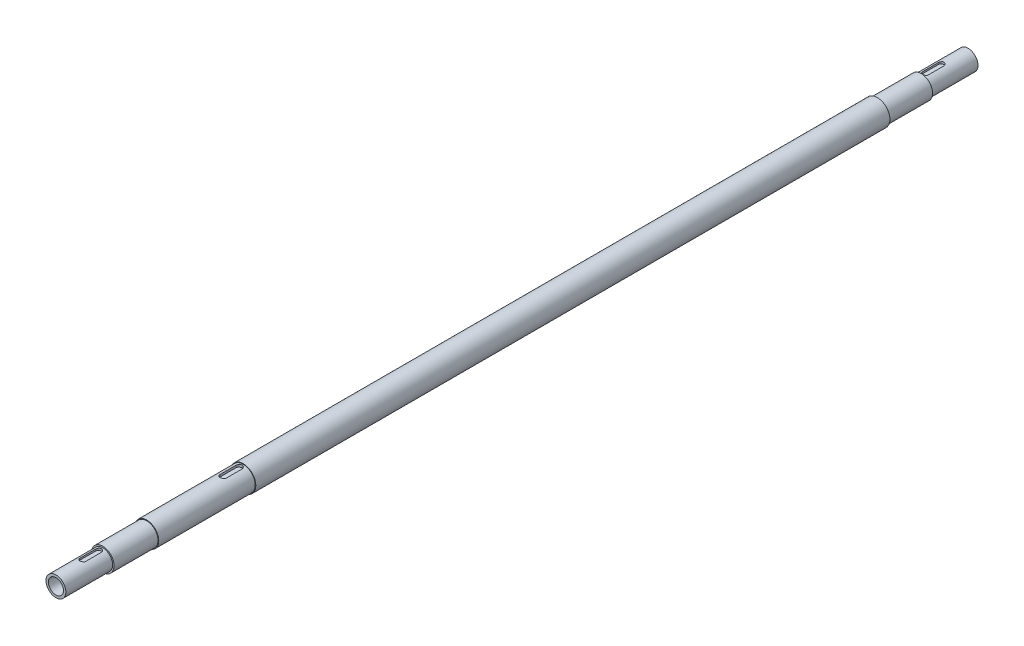
from build123d import *

# Parameters (mm, degrees)
SKETCH1_R           = 44.5
BOSS_EXTRUDE1_DEPTH = 3215
CUT_EXTRUDE1_START  = -165
SKETCH2_R           = 44.5
SKETCH2_R_2         = 37.5
CUT_EXTRUDE1_DEPTH  = 165
CUT_EXTRUDE2_START  = -155
SKETCH3_R           = 44.5
SKETCH3_R_2         = 40
CUT_EXTRUDE2_DEPTH  = 155
CUT_EXTRUDE3_START  = -340
SKETCH4_R           = 44.5
SKETCH4_R_2         = 42.5
CUT_EXTRUDE3_DEPTH  = 340
SKETCH8_R           = 26.5
CUT_EXTRUDE7_DEPTH  = 3216.615881911
CUT_EXTRUDE8_START  = -165
SKETCH10_R          = 37.5
SKETCH10_R_2        = 35
CUT_EXTRUDE8_DEPTH  = 165
CUT_EXTRUDE9_DEPTH  = 7.5
CUT_EXTRUDE10_DEPTH = 9


with BuildPart() as part:
    # Sketch1 → Boss-Extrude1 (new body)
    with BuildSketch(Plane.XY):
        with Locations(Location((0, 0, 0), (0, 0, 180))):
            Circle(SKETCH1_R)
    extrude(amount=BOSS_EXTRUDE1_DEPTH)

    # Sketch2 → Cut-Extrude1 (cut)
    with BuildSketch(Plane.XY.offset(3215).offset(CUT_EXTRUDE1_START)):
        with Locations(Location((0, 0, 0), (0, 0, 180))):
            Circle(SKETCH2_R)
        Circle(SKETCH2_R_2, mode=Mode.SUBTRACT)
    cut_extrude1 = extrude(amount=CUT_EXTRUDE1_DEPTH, mode=Mode.SUBTRACT)

    # Sketch3 → Cut-Extrude2 (cut)
    with BuildSketch(Plane.XY.offset(3050).offset(CUT_EXTRUDE2_START)):
        with Locations(Location((0, 0, 0), (0, 0, 180))):
            Circle(SKETCH3_R)
        Circle(SKETCH3_R_2, mode=Mode.SUBTRACT)
    cut_extrude2 = extrude(amount=CUT_EXTRUDE2_DEPTH, mode=Mode.SUBTRACT)

    # Sketch4 → Cut-Extrude3 (cut)
    with BuildSketch(Plane.XY.offset(2895).offset(CUT_EXTRUDE3_START)):
        with Locations(Location((0, 0, 0), (0, 0, 180))):
            Circle(SKETCH4_R)
        Circle(SKETCH4_R_2, mode=Mode.SUBTRACT)
    extrude(amount=CUT_EXTRUDE3_DEPTH, mode=Mode.SUBTRACT)

    # Sketch8 → Cut-Extrude7 (cut, through all)
    with BuildSketch(Plane.XY.offset(3215)):
        Circle(SKETCH8_R)
    extrude(amount=-CUT_EXTRUDE7_DEPTH, mode=Mode.SUBTRACT)

    # Sketch10 → Cut-Extrude8 (cut)
    with BuildSketch(Plane.XY.offset(3215).offset(CUT_EXTRUDE8_START)):
        Circle(SKETCH10_R)
        Circle(SKETCH10_R_2, mode=Mode.SUBTRACT)
    cut_extrude8 = extrude(amount=CUT_EXTRUDE8_DEPTH, mode=Mode.SUBTRACT)

    # Mirror1: Cut-Extrude1, Cut-Extrude2, Cut-Extrude8 across plane
    add(cut_extrude1.mirror(Plane.XY.offset(1607.5)), mode=Mode.SUBTRACT)
    add(cut_extrude2.mirror(Plane.XY.offset(1607.5)), mode=Mode.SUBTRACT)
    add(cut_extrude8.mirror(Plane.XY.offset(1607.5)), mode=Mode.SUBTRACT)

    # Sketch11 → Cut-Extrude9 (cut)
    with BuildSketch(Plane(origin=(0, 35, 0), x_dir=(1, 0, 0), z_dir=(0, 1, 0))):
        with BuildLine():
            Line((10, -3065), (10, -3120))
            ThreePointArc((10, -3120), (0, -3130), (-10, -3120))
            Line((-10, -3120), (-10, -3065))
            ThreePointArc((-10, -3065), (0, -3055), (10, -3065))
        make_face()
    cut_extrude9 = extrude(amount=-CUT_EXTRUDE9_DEPTH, mode=Mode.SUBTRACT)

    # Mirror2: Cut-Extrude9 across plane
    add(cut_extrude9.mirror(Plane.XY.offset(1607.5)), mode=Mode.SUBTRACT)

    # Sketch12 → Cut-Extrude10 (cut)
    with BuildSketch(Plane(origin=(0, 42.5, 0), x_dir=(1, 0, 0), z_dir=(0, 1, 0))):
        with BuildLine():
            Line((11, -2570), (11, -2625))
            ThreePointArc((11, -2625), (0, -2636), (-11, -2625))
            Line((-11, -2625), (-11, -2570))
            ThreePointArc((-11, -2570), (0, -2559), (11, -2570))
        make_face()
    extrude(amount=-CUT_EXTRUDE10_DEPTH, mode=Mode.SUBTRACT)


solid = part.part
